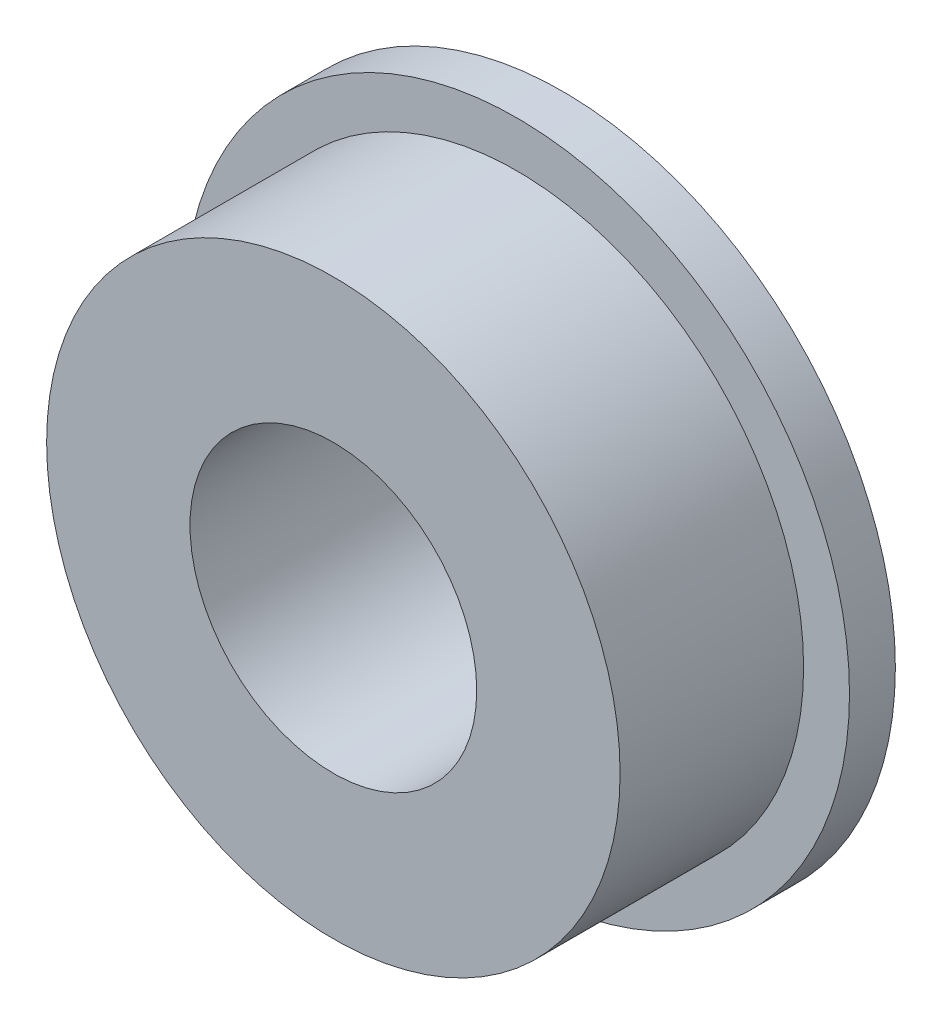
SolidWorks part; units mm, degrees
material "钴"
ref_plane "前视基准面" through (0, 0, 0) normal (0, 0, 1) x (1, 0, 0)
ref_plane "上视基准面" through (0, 0, 0) normal (0, 1, 0) x (1, 0, 0)
ref_plane "右视基准面" through (0, 0, 0) normal (1, 0, 0) x (0, 0, -1)
other "Configuration Table"
sketch "草图1" plane through (0, 0, 0) normal (0, 0, 1) x (1, 0, 0)
  circle A0 centre (0, 0) radius 5.8
  circle A1 centre (0, 0) radius 2.5
  dimension "D1" = 5
  dimension "D2" = 11.6
extrude "凸台-拉伸1" add sketch "草图1" along normal blind 0.8
sketch "草图2" plane through (0, 0, 0.8) normal (0, 0, 1) x (1, 0, 0)
  circle A0 centre (0, 0) radius 5
  circle A1 centre (0, 0) radius 2.5 construction
  circle A2 centre (0, 0) radius 2.5
  dimension "D1" = 10
extrude "凸台-拉伸2" add sketch "草图2" along normal blind 3.2
